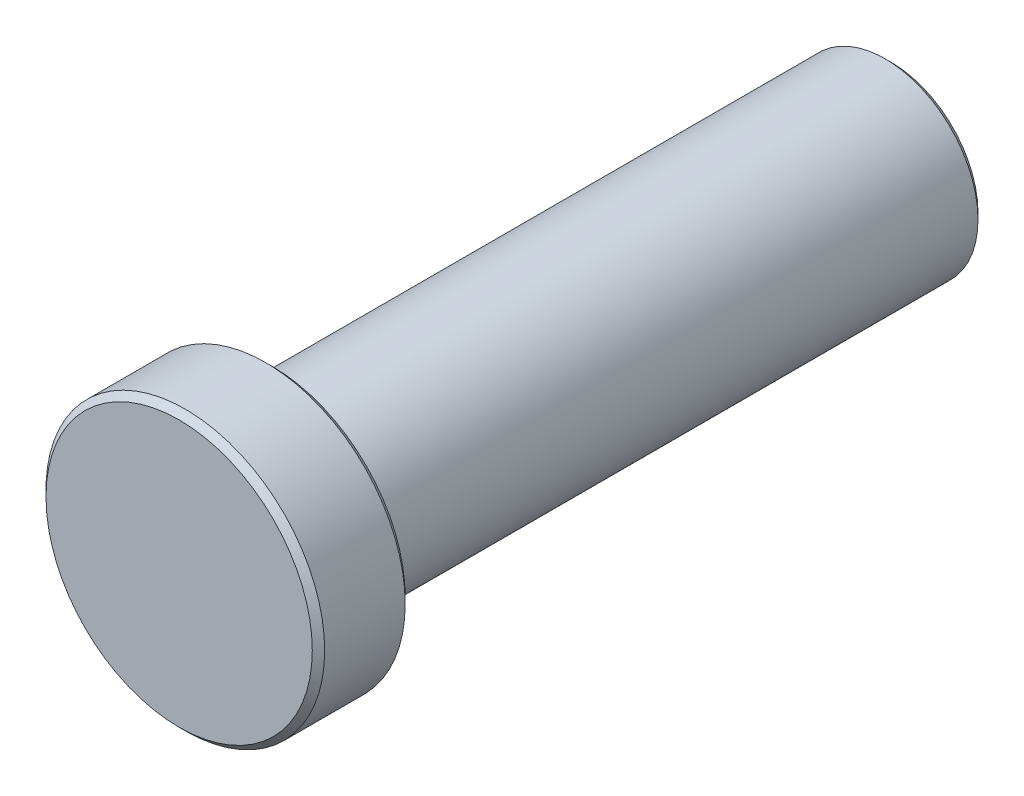
SolidWorks part; units mm, degrees
ref_plane "Front Plane" through (0, 0, 0) normal (0, 0, 1) x (1, 0, 0)
ref_plane "Top Plane" through (0, 0, 0) normal (0, 1, 0) x (1, 0, 0)
ref_plane "Right Plane" through (0, 0, 0) normal (1, 0, 0) x (0, 0, -1)
sketch "Sketch1" plane through (0, 0, 0) normal (0, 0, 1) x (1, 0, 0)
  circle A0 centre (0, 0) radius 3
  dimension "D1" = 6
extrude "Boss-Extrude1" add sketch "Sketch1" along normal blind 20
sketch "Sketch2" plane through (0, 0, 20) normal (0, 0, 1) x (1, 0, 0)
  circle A0 centre (0, 0) radius 4.5
  dimension "D1" = 9
extrude "Boss-Extrude2" add sketch "Sketch2" along normal blind 3
chamfer "Chamfer1" distance 0.2 angle 45 3 edges at (4.5, 0, 23) (4.5, 0, 20) (3, 0, 0)
